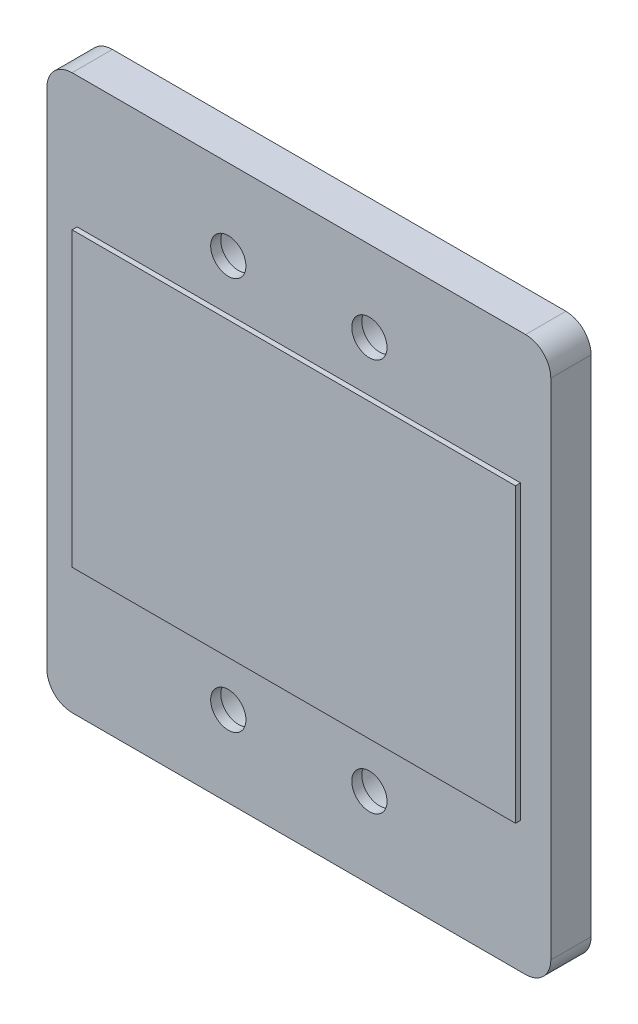
SolidWorks part; units mm, degrees
ref_plane "Front Plane" through (0, 0, 0) normal (0, 0, 1) x (1, 0, 0)
ref_plane "Top Plane" through (0, 0, 0) normal (0, 1, 0) x (1, 0, 0)
ref_plane "Right Plane" through (0, 0, 0) normal (1, 0, 0) x (0, 0, -1)
sketch "Sketch1" plane through (0, 0, 0) normal (0, 0, 1) x (1, 0, 0)
  line L1 (-45, -55) -> (45, -55)
  line L2 (-50, -50) -> (-50, 50)
  line L3 (-45, 55) -> (45, 55)
  line L4 (50, -50) -> (50, 50)
  line L5 (-50, -55) -> (50, 55) construction
  line L6 (-50, 55) -> (50, -55) construction
  arc A0 (-45, -55) -> (-50, -50) centre (-45, -50) cw
  arc A1 (45, -55) -> (50, -50) centre (45, -50) ccw
  arc A2 (45, 55) -> (50, 50) centre (45, 50) cw
  arc A3 (-50, 50) -> (-45, 55) centre (-45, 50) cw
  point P0 (0, 0)
  dimension "D3" = 5
  dimension "D1" = 110
  dimension "D2" = 100
extrude "Boss-Extrude1" add sketch "Sketch1" along normal blind 8
sketch "Sketch2" plane through (0, 0, 8) normal (0, 0, 1) x (1, 0, 0)
  line L1 (-44, -29) -> (44, -29)
  line L2 (-44, -29) -> (-44, 29)
  line L3 (-44, 29) -> (44, 29)
  line L4 (44, -29) -> (44, 29)
  line L5 (-44, -29) -> (44, 29) construction
  line L6 (-44, 29) -> (44, -29) construction
  point P0 (0, 0)
  dimension "D1" = 58
  dimension "D2" = 88
extrude "Boss-Extrude2" add sketch "Sketch2" along normal blind 1
sketch "Sketch4" plane through (0, 0, 0) normal (0, 0, -1) x (-1, 0, 0)
  line L0 (0, 0) -> (50, 0) construction
  line L1 (50, 50) -> (50, -50) construction
  circle A0 centre (-14, -39) radius 6
  circle A1 centre (14, -39) radius 6
  circle A2 centre (14, 39) radius 6
  circle A3 centre (-14, 39) radius 6
  dimension "D3" = 12
  dimension "D1" = 14
  dimension "D2" = 14
  dimension "D4" = 39
extrude "Cut-Extrude1" cut sketch "Sketch4" against normal blind 6
sketch "Sketch5" plane through (0, 0, 6) normal (0, 0, -1) x (-1, 0, 0)
  line L0 (0, 0) -> (50, 0) construction
  line L1 (50, 50) -> (50, -50) construction
  circle A0 centre (-14, 39) radius 3.5
  circle A1 centre (14, 39) radius 3.5
  circle A2 centre (14, -39) radius 3.5
  circle A3 centre (-14, -39) radius 3.5
  dimension "D1" = 7
extrude "Cut-Extrude2" cut sketch "Sketch5" against normal blind 6
